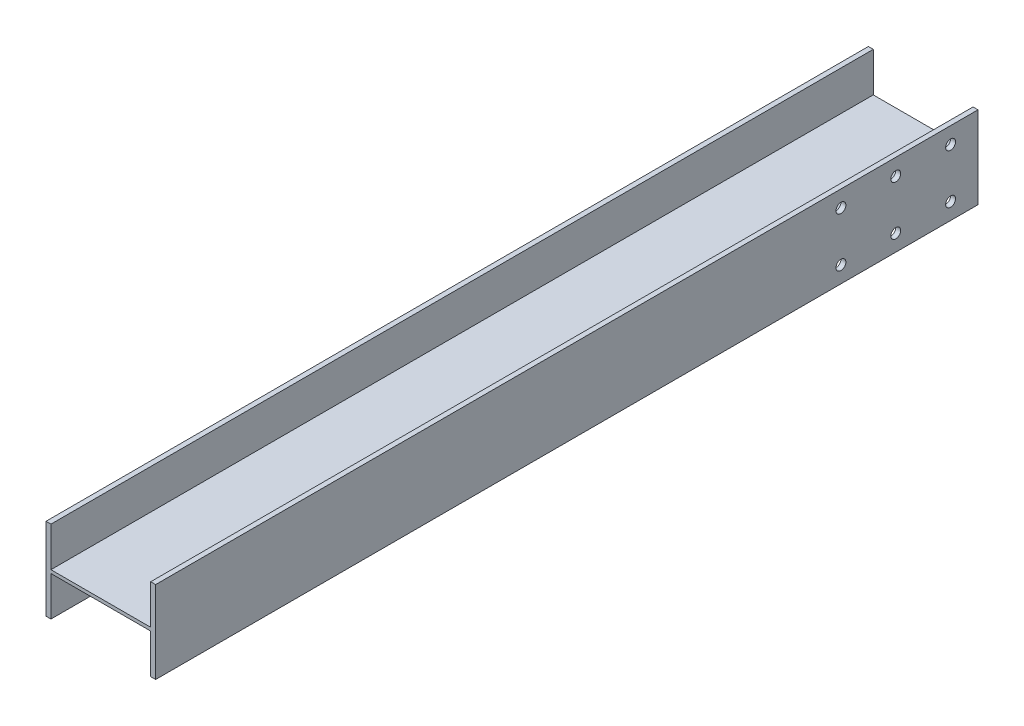
from build123d import *

# Parameters (mm, degrees)
BOSS_EXTRUDE1_DEPTH = 1500
SKETCH2_R           = 9
CUT_EXTRUDE1_DEPTH  = 1500


with BuildPart() as part:
    # Sketch1 → Boss-Extrude1 (new body)
    with BuildSketch(Plane.XY):
        Polygon((-91, -75), (-100, -75), (-100, 75), (-91, 75), (-91, 3), (91, 3), (91, 75), (100, 75), (100, -75), (91, -75), (91, -3), (-91, -3), align=None)
    extrude(amount=BOSS_EXTRUDE1_DEPTH)

    # Sketch2 → Cut-Extrude1 (cut)
    with BuildSketch(Plane.ZY.offset(-91)):
        with Locations((50, -45)):
            Circle(SKETCH2_R)
        with Locations((150, -45)):
            Circle(SKETCH2_R)
        with Locations((250, -45)):
            Circle(SKETCH2_R)
        with Locations(Location((250, 45, 0), (0, 0, 270))):
            Circle(SKETCH2_R)
        with Locations(Location((150, 45, 0), (0, 0, 270))):
            Circle(SKETCH2_R)
        with Locations(Location((50, 45, 0), (0, 0, 270))):
            Circle(SKETCH2_R)
    extrude(amount=-CUT_EXTRUDE1_DEPTH, mode=Mode.SUBTRACT)


solid = part.part
